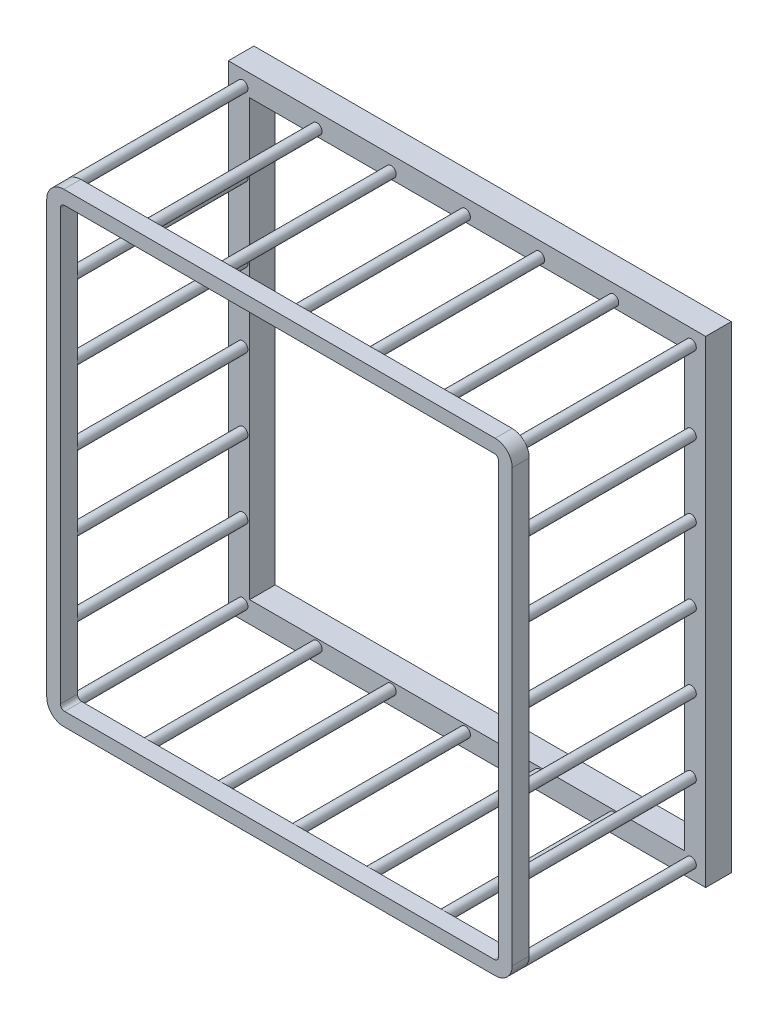
from build123d import *

# Parameters (mm, degrees)
SKETCH1_W           = 560
SKETCH1_H           = 560
SKETCH1_W_2         = 510
SKETCH1_H_2         = 510
BOSS_EXTRUDE1_DEPTH = 30
SKETCH2_R           = 6
BOSS_EXTRUDE2_DEPTH = 200
BOSS_EXTRUDE3_DEPTH = 20


with BuildPart() as part:
    # Sketch1 → Boss-Extrude1 (new body)
    with BuildSketch(Plane.XY):
        with Locations((280, 280)):
            Rectangle(SKETCH1_W, SKETCH1_H)
        with Locations((280, 280)):
            Rectangle(SKETCH1_W_2, SKETCH1_H_2, mode=Mode.SUBTRACT)
    extrude(amount=BOSS_EXTRUDE1_DEPTH)

    # Sketch2 → Boss-Extrude2 (add)
    with BuildSketch(Plane.XY.offset(30)):
        with Locations(Location((17, 543, 0), (0, 0, 180))):
            Circle(SKETCH2_R)
        with Locations(Location((17, 17, 0), (0, 0, 180))):
            Circle(SKETCH2_R)
        with Locations(Location((543, 17, 0), (0, 0, 180))):
            Circle(SKETCH2_R)
        with Locations(Location((543, 543, 0), (0, 0, 180))):
            Circle(SKETCH2_R)
        with Locations(Location((104, 543, 0), (0, 0, 180))):
            Circle(SKETCH2_R)
        with Locations(Location((104, 17, 0), (0, 0, 180))):
            Circle(SKETCH2_R)
        with Locations(Location((191, 543, 0), (0, 0, 180))):
            Circle(SKETCH2_R)
        with Locations(Location((191, 17, 0), (0, 0, 180))):
            Circle(SKETCH2_R)
        with Locations(Location((278, 543, 0), (0, 0, 180))):
            Circle(SKETCH2_R)
        with Locations(Location((278, 17, 0), (0, 0, 180))):
            Circle(SKETCH2_R)
        with Locations(Location((365, 543, 0), (0, 0, 180))):
            Circle(SKETCH2_R)
        with Locations(Location((365, 17, 0), (0, 0, 180))):
            Circle(SKETCH2_R)
        with Locations(Location((452, 543, 0), (0, 0, 180))):
            Circle(SKETCH2_R)
        with Locations(Location((452, 17, 0), (0, 0, 180))):
            Circle(SKETCH2_R)
        with Locations(Location((17, 104, 0), (0, 0, 180))):
            Circle(SKETCH2_R)
        with Locations(Location((543, 104, 0), (0, 0, 180))):
            Circle(SKETCH2_R)
        with Locations(Location((17, 191, 0), (0, 0, 180))):
            Circle(SKETCH2_R)
        with Locations(Location((543, 191, 0), (0, 0, 180))):
            Circle(SKETCH2_R)
        with Locations(Location((17, 278, 0), (0, 0, 180))):
            Circle(SKETCH2_R)
        with Locations(Location((543, 278, 0), (0, 0, 180))):
            Circle(SKETCH2_R)
        with Locations(Location((17, 365, 0), (0, 0, 180))):
            Circle(SKETCH2_R)
        with Locations(Location((543, 365, 0), (0, 0, 180))):
            Circle(SKETCH2_R)
        with Locations(Location((17, 452, 0), (0, 0, 180))):
            Circle(SKETCH2_R)
        with Locations(Location((543, 452, 0), (0, 0, 180))):
            Circle(SKETCH2_R)
    extrude(amount=BOSS_EXTRUDE2_DEPTH)

    # Sketch3 → Boss-Extrude3 (add)
    with BuildSketch(Plane.XY.offset(230)):
        with BuildLine():
            Line((7, 533), (7, 27))
            ThreePointArc((7, 27), (12.857864376, 12.857864376), (27, 7))
            Line((27, 7), (533, 7))
            ThreePointArc((533, 7), (547.142135624, 12.857864376), (553, 27))
            Line((553, 27), (553, 533))
            ThreePointArc((553, 533), (547.142135624, 547.142135624), (533, 553))
            Line((533, 553), (27, 553))
            ThreePointArc((27, 553), (12.857864376, 547.142135624), (7, 533))
        make_face()
        with BuildLine():
            Line((23, 532), (23, 28))
            ThreePointArc((23, 28), (24.464466094, 24.464466094), (28, 23))
            Line((28, 23), (532, 23))
            ThreePointArc((532, 23), (535.535533906, 24.464466094), (537, 28))
            Line((537, 28), (537, 532))
            ThreePointArc((537, 532), (535.535533906, 535.535533906), (532, 537))
            Line((532, 537), (28, 537))
            ThreePointArc((28, 537), (24.464466094, 535.535533906), (23, 532))
        make_face(mode=Mode.SUBTRACT)
    extrude(amount=BOSS_EXTRUDE3_DEPTH)


solid = part.part
